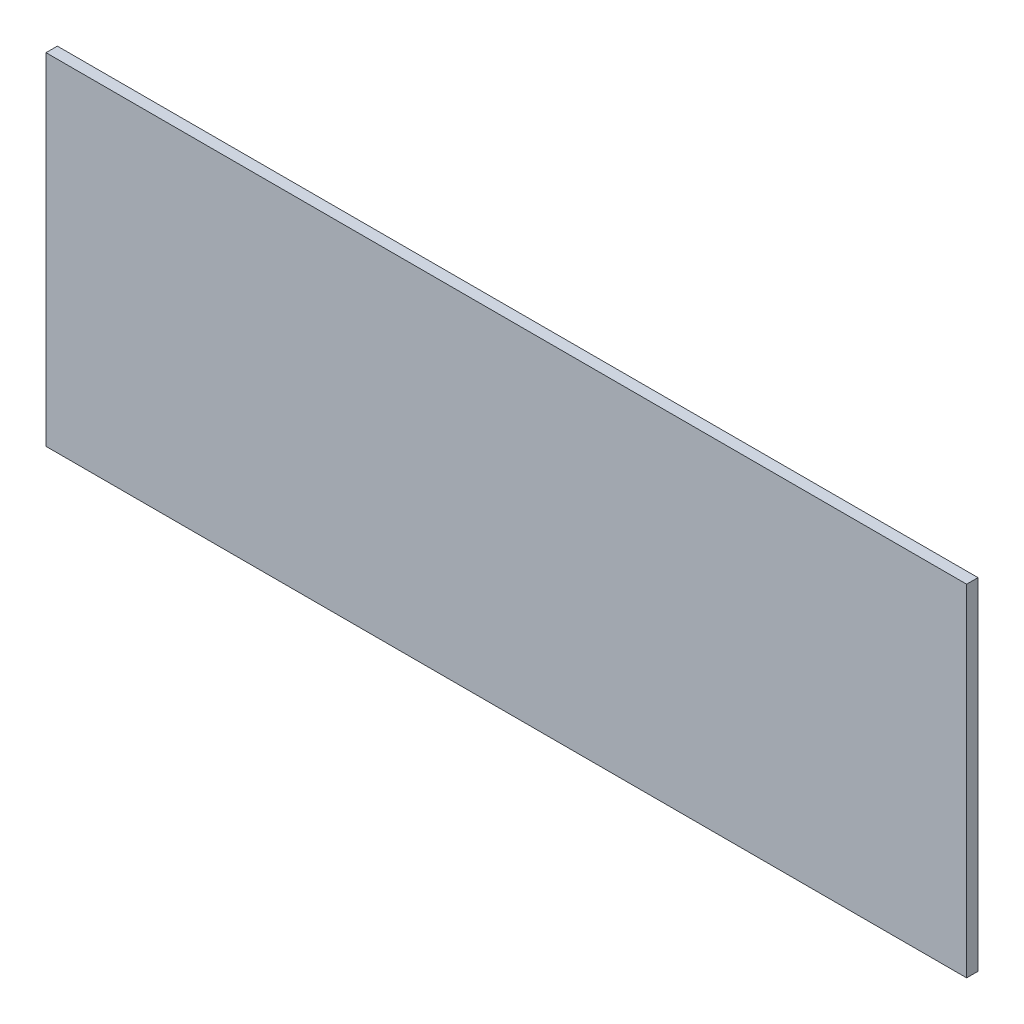
SolidWorks part; units mm, degrees
ref_plane "前视基准面" through (0, 0, 0) normal (0, 0, 1) x (1, 0, 0)
ref_plane "上视基准面" through (0, 0, 0) normal (0, 1, 0) x (1, 0, 0)
ref_plane "右视基准面" through (0, 0, 0) normal (1, 0, 0) x (0, 0, -1)
sketch "草图1" plane through (0, 0, 0) normal (0, 0, 1) x (1, 0, 0)
  line L1 (-202.5, 75) -> (202.5, 75)
  line L2 (-202.5, 75) -> (-202.5, -75)
  line L3 (-202.5, -75) -> (202.5, -75)
  line L4 (202.5, 75) -> (202.5, -75)
  line L5 (-202.5, 75) -> (202.5, -75) construction
  line L6 (-202.5, -75) -> (202.5, 75) construction
  point P0 (0, 0)
  dimension "D1" = 405
  dimension "D2" = 150
extrude "凸台-拉伸1" add sketch "草图1" along normal blind 5
